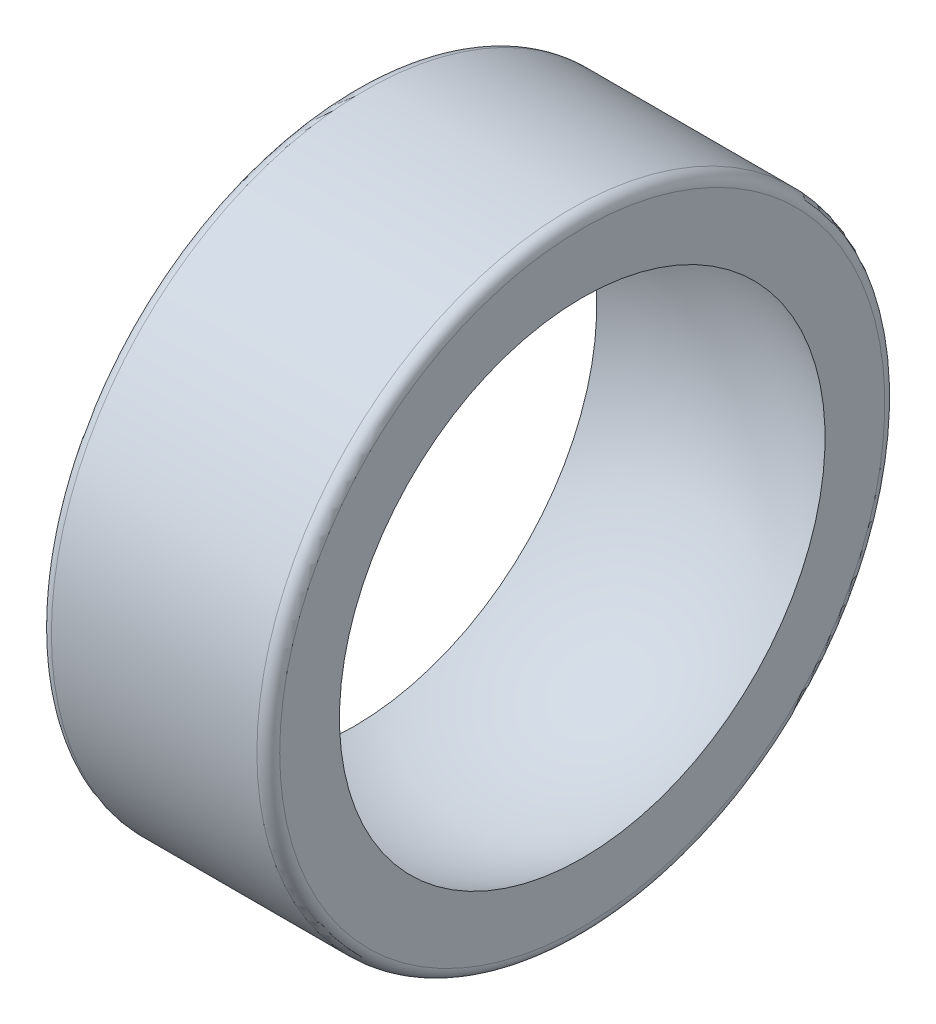
from build123d import *

# Parameters (mm, degrees)
FILLET_1_R = 1


with BuildPart() as part:
    # 草图1 → 旋转1 (revolve)
    with BuildSketch(Plane.XY, mode=Mode.PRIVATE) as revolve_1_sk:
        with BuildLine():
            Line((-10, 27.5), (-10, 21.266170318))
            ThreePointArc((-10, 21.266170318), (0, 23.5), (10, 21.266170318))
            Line((10, 21.266170318), (10, 27.5))
            Line((10, 27.5), (-10, 27.5))
        make_face()
    revolve(revolve_1_sk.sketch.rotate(Axis((-48.231282768, 0, 0), (1, 0, 0)), 90), axis=Axis((-48.231282768, 0, 0), (1, 0, 0)))

    # 圆角1
    fillet_1_edges = [part.edges().sort_by_distance(p)[0] for p in [
        (10, 0, -27.5),
        (-10, 0, -27.5),
    ]]
    fillet(fillet_1_edges, radius=FILLET_1_R)


solid = part.part
